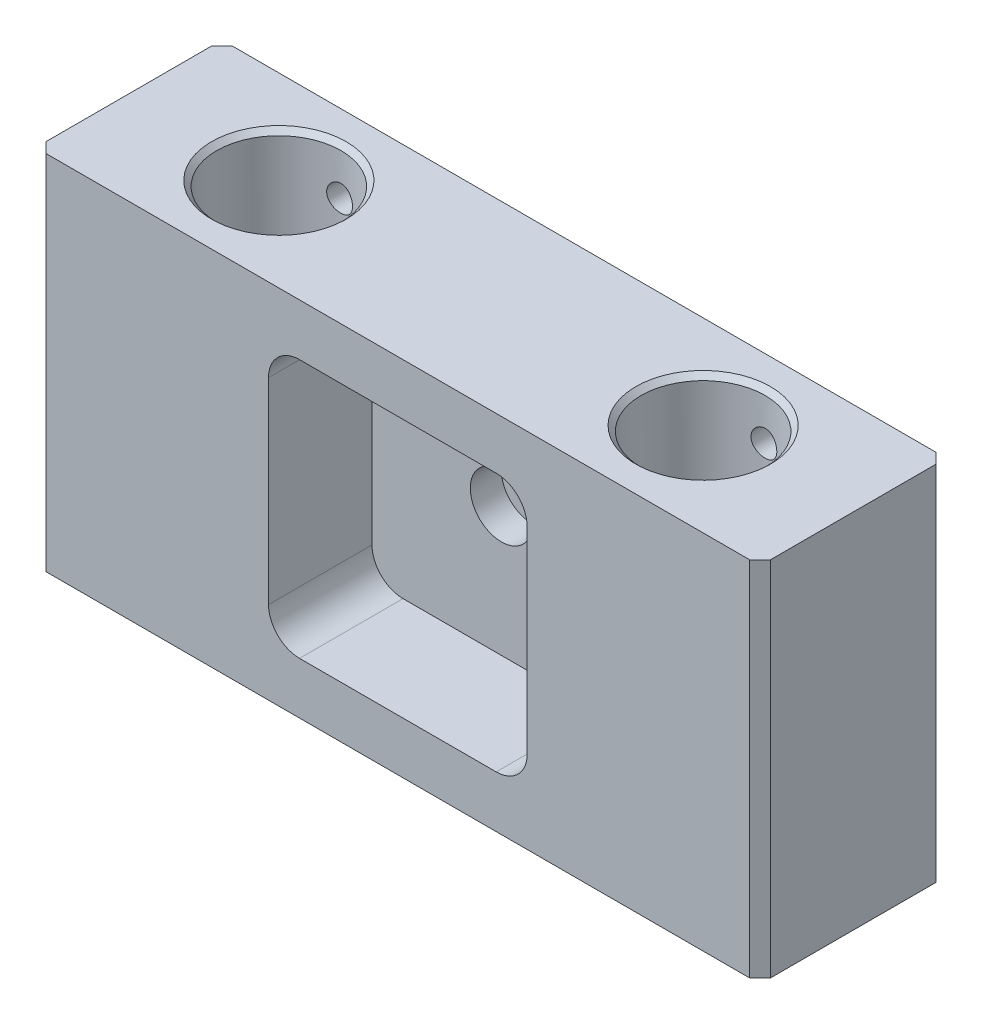
from build123d import *

# Parameters (mm, degrees)
SKETCH1_W                               = 70
SKETCH1_H                               = 35
BOSS_EXTRUDE1_DEPTH                     = 9
CUT_EXTRUDE1_DEPTH                      = 10
SKETCH3_R                               = 6
CUT_EXTRUDE2_DEPTH                      = 51.309044912
M3_TAPPED_HOLE1_REACH                   = 45.073
M3_TAPPED_HOLE1_BORE_R                  = 1.25
CBORE_FOR_M3_HEX_HEAD_BOLT1_D           = 3.5
CBORE_FOR_M3_HEX_HEAD_BOLT1_CBORE_D     = 6
CBORE_FOR_M3_HEX_HEAD_BOLT1_CBORE_DEPTH = 3
CUT_EXTRUDE3_START                      = -3
SKETCH9_R                               = 3
CUT_EXTRUDE3_DEPTH                      = 3
CHAMFER1_SIZE                           = 1
CHAMFER2_SIZE                           = 0.5


with BuildPart() as part:
    # Sketch1 → Boss-Extrude1 (new, symmetric)
    with BuildSketch(Plane.XY):
        Rectangle(SKETCH1_W, SKETCH1_H)
    extrude(amount=BOSS_EXTRUDE1_DEPTH, both=True)

    # Sketch2 → Cut-Extrude1 (cut)
    with BuildSketch(Plane.XY.offset(9)):
        with BuildLine():
            Line((-9.5, 12.5), (9.5, 12.5))
            ThreePointArc((9.5, 12.5), (11.621320344, 11.621320344), (12.5, 9.5))
            Line((12.5, 9.5), (12.5, -9.5))
            ThreePointArc((12.5, -9.5), (11.621320344, -11.621320344), (9.5, -12.5))
            Line((9.5, -12.5), (-9.5, -12.5))
            ThreePointArc((-9.5, -12.5), (-11.621320344, -11.621320344), (-12.5, -9.5))
            Line((-12.5, -9.5), (-12.5, 9.5))
            ThreePointArc((-12.5, 9.5), (-11.621320344, 11.621320344), (-9.5, 12.5))
        make_face()
    extrude(amount=-CUT_EXTRUDE1_DEPTH, mode=Mode.SUBTRACT)

    # Sketch3 → Cut-Extrude2 (cut, through all)
    with BuildSketch(Plane(origin=(0, 17.5, 0), x_dir=(1, 0, 0), z_dir=(0, 1, 0))):
        with Locations(Location((-20.5, 0, 0), (0, 0, 270))):
            Circle(SKETCH3_R)
        with Locations(Location((20.5, 0, 0), (0, 0, 270))):
            Circle(SKETCH3_R)
    extrude(amount=-CUT_EXTRUDE2_DEPTH, mode=Mode.SUBTRACT)

    # M3 Tapped Hole1 bore → M3 Tapped Hole1 (cut, up to next)
    with BuildSketch(Plane(origin=(0, 0, -9), x_dir=(-1, 0, 0), z_dir=(0, 0, -1)), mode=Mode.PRIVATE) as m3_tapped_hole1_sk1:
        with Locations((-20.5, 13)):
            Circle(M3_TAPPED_HOLE1_BORE_R)
    m3_tapped_hole1_tool1 = extrude(m3_tapped_hole1_sk1.sketch, amount=-M3_TAPPED_HOLE1_REACH, mode=Mode.PRIVATE) & part.part
    # M3 Tapped Hole1 bore → M3 Tapped Hole1 (cut, up to next)
    with BuildSketch(Plane(origin=(0, 0, -9), x_dir=(-1, 0, 0), z_dir=(0, 0, -1)), mode=Mode.PRIVATE) as m3_tapped_hole1_sk2:
        with Locations((-20.5, -13)):
            Circle(M3_TAPPED_HOLE1_BORE_R)
    m3_tapped_hole1_tool2 = extrude(m3_tapped_hole1_sk2.sketch, amount=-M3_TAPPED_HOLE1_REACH, mode=Mode.PRIVATE) & part.part
    # M3 Tapped Hole1 bore → M3 Tapped Hole1 (cut, up to next)
    with BuildSketch(Plane(origin=(0, 0, -9), x_dir=(-1, 0, 0), z_dir=(0, 0, -1)), mode=Mode.PRIVATE) as m3_tapped_hole1_sk3:
        with Locations((20.5, -13)):
            Circle(M3_TAPPED_HOLE1_BORE_R)
    m3_tapped_hole1_tool3 = extrude(m3_tapped_hole1_sk3.sketch, amount=-M3_TAPPED_HOLE1_REACH, mode=Mode.PRIVATE) & part.part
    # M3 Tapped Hole1 bore → M3 Tapped Hole1 (cut, up to next)
    with BuildSketch(Plane(origin=(0, 0, -9), x_dir=(-1, 0, 0), z_dir=(0, 0, -1)), mode=Mode.PRIVATE) as m3_tapped_hole1_sk4:
        with Locations((20.5, 13)):
            Circle(M3_TAPPED_HOLE1_BORE_R)
    m3_tapped_hole1_tool4 = extrude(m3_tapped_hole1_sk4.sketch, amount=-M3_TAPPED_HOLE1_REACH, mode=Mode.PRIVATE) & part.part
    add(m3_tapped_hole1_tool1.solids().sort_by_distance((20.5, 13, -9))[0], mode=Mode.SUBTRACT)
    add(m3_tapped_hole1_tool2.solids().sort_by_distance((20.5, -13, -9))[0], mode=Mode.SUBTRACT)
    add(m3_tapped_hole1_tool3.solids().sort_by_distance((-20.5, -13, -9))[0], mode=Mode.SUBTRACT)
    add(m3_tapped_hole1_tool4.solids().sort_by_distance((-20.5, 13, -9))[0], mode=Mode.SUBTRACT)

    # CBORE for M3 Hex Head Bolt1 (through all)
    with Locations(Plane(origin=(-21.223251094, -7.58728159, -1), x_dir=(1, 0, 0), z_dir=(0, 0, 1))):
        with Locations((21.223251094, 7.58728159)):
            CounterBoreHole(CBORE_FOR_M3_HEX_HEAD_BOLT1_D / 2, CBORE_FOR_M3_HEX_HEAD_BOLT1_CBORE_D / 2, CBORE_FOR_M3_HEX_HEAD_BOLT1_CBORE_DEPTH)

    # Sketch9 → Cut-Extrude3 (cut)
    with BuildSketch(Plane(origin=(0, 0, -9), x_dir=(-1, 0, 0), z_dir=(0, 0, -1)).offset(CUT_EXTRUDE3_START)):
        with Locations(Location((0, 0, 0), (0, 0, 180))):
            Circle(SKETCH9_R)
    extrude(amount=CUT_EXTRUDE3_DEPTH, mode=Mode.SUBTRACT)

    # Chamfer1
    chamfer1_edges = [part.edges().sort_by_distance(p)[0] for p in [
        (-35, 0, 9),
        (35, 0, 9),
        (-35, 0, -9),
        (35, 0, -9),
    ]]
    chamfer(chamfer1_edges, length=CHAMFER1_SIZE)

    # Chamfer2
    chamfer2_edges = [part.edges().sort_by_distance(p)[0] for p in [
        (-20.5, -17.5, -6),
        (-20.5, 17.5, -6),
        (20.5, -17.5, -6),
        (20.5, 17.5, -6),
    ]]
    chamfer(chamfer2_edges, length=CHAMFER2_SIZE)


solid = part.part
